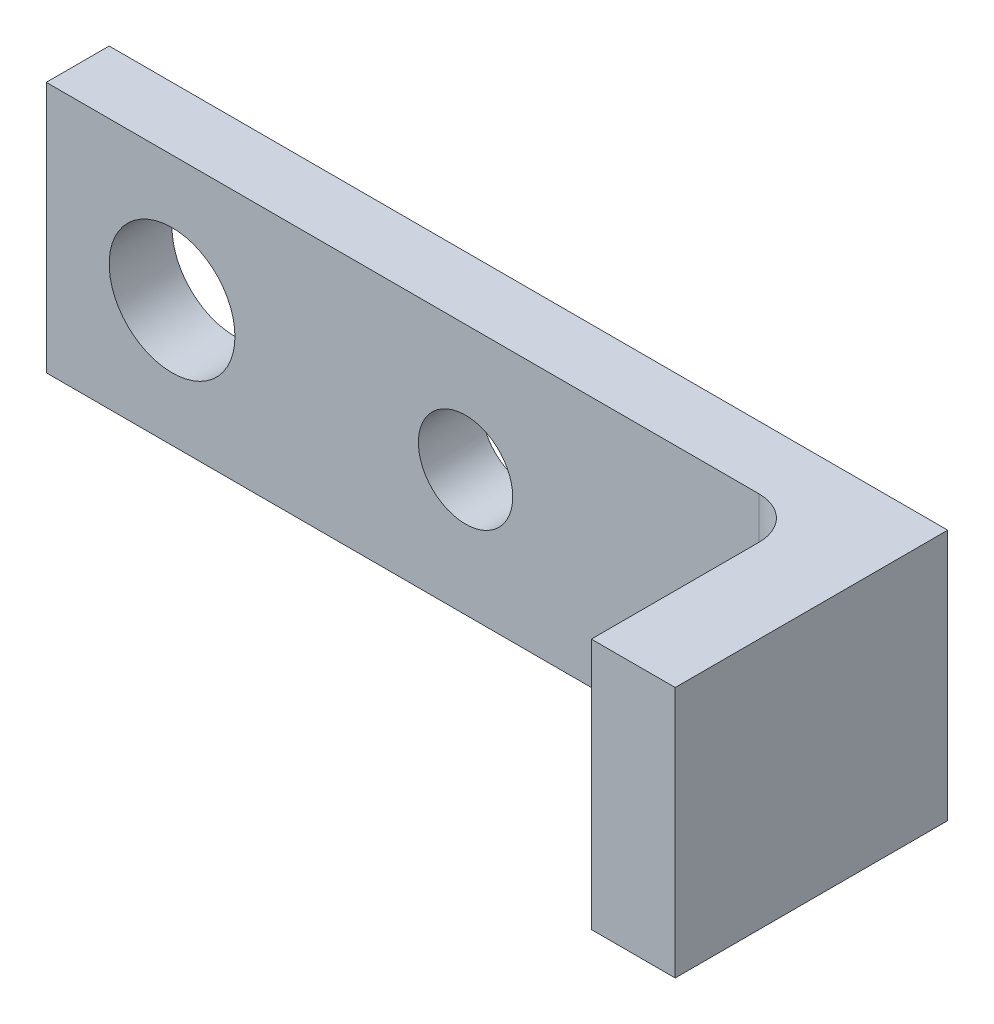
from build123d import *

# Parameters (mm, degrees)
SKETCH1_W           = 40
SKETCH1_H           = 12
SKETCH1_R           = 2.25
SKETCH1_R_2         = 3
BOSS_EXTRUDE1_DEPTH = 3
SKETCH2_W           = 4
SKETCH2_H           = 12
BOSS_EXTRUDE2_DEPTH = 10
FILLET1_R           = 2


with BuildPart() as part:
    # Sketch1 → Boss-Extrude1 (new body)
    with BuildSketch(Plane.XY):
        with Locations((20, 6)):
            Rectangle(SKETCH1_W, SKETCH1_H)
        with Locations((20, 6)):
            Circle(SKETCH1_R, mode=Mode.SUBTRACT)
        with Locations((6, 6)):
            Circle(SKETCH1_R_2, mode=Mode.SUBTRACT)
    extrude(amount=BOSS_EXTRUDE1_DEPTH)

    # Sketch2 → Boss-Extrude2 (add)
    with BuildSketch(Plane.XY.offset(3)):
        with Locations((38, 6)):
            Rectangle(SKETCH2_W, SKETCH2_H)
    extrude(amount=BOSS_EXTRUDE2_DEPTH)

    # Fillet1
    fillet1_edges = [part.edges().sort_by_distance(p)[0] for p in [
        (36, 6, 3),
    ]]
    fillet(fillet1_edges, radius=FILLET1_R)


solid = part.part
